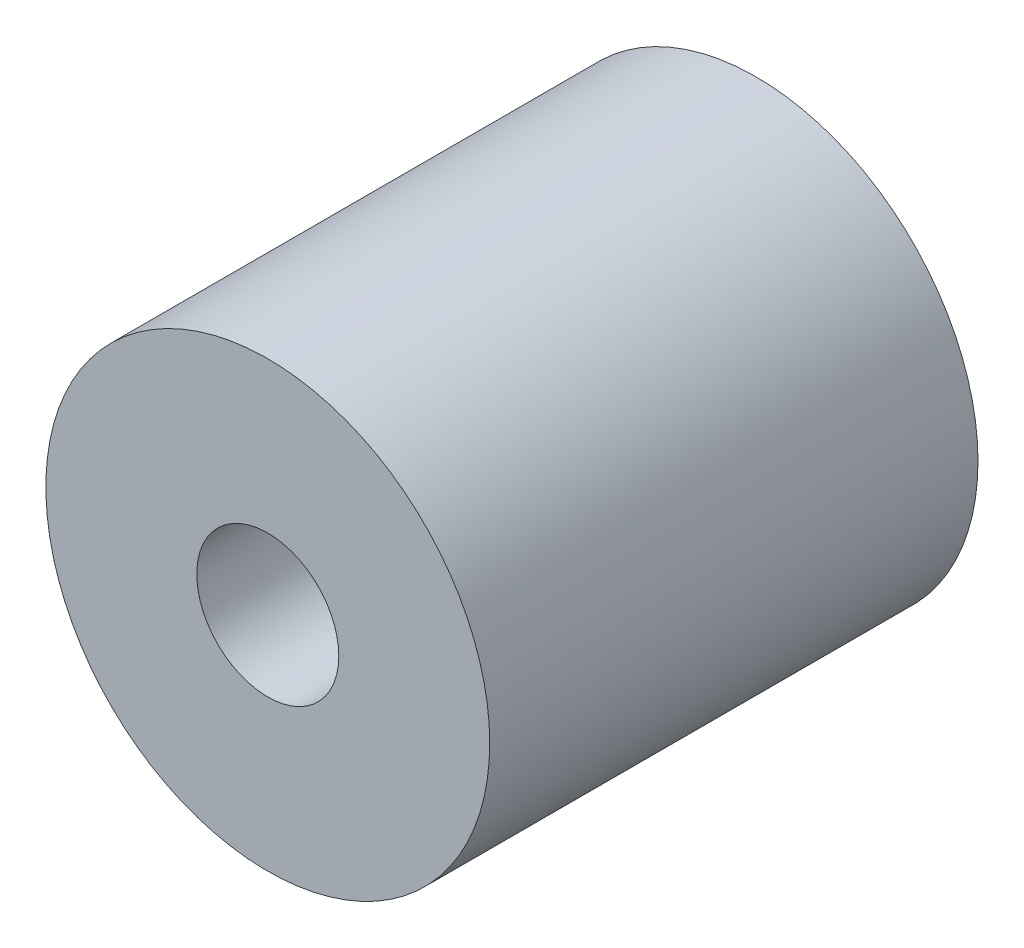
SolidWorks part; units mm, degrees
ref_plane "前视基准面" through (0, 0, 0) normal (0, 0, 1) x (1, 0, 0)
ref_plane "上视基准面" through (0, 0, 0) normal (0, 1, 0) x (1, 0, 0)
ref_plane "右视基准面" through (0, 0, 0) normal (1, 0, 0) x (0, 0, -1)
other "Configuration Table"
sketch "草图1" plane through (0, 0, 0) normal (0, 0, 1) x (1, 0, 0)
  circle A0 centre (0, 0) radius 10
  circle A1 centre (0, 0) radius 3.2
  point P0 (0, 0)
  dimension "D1" = 6.4
  dimension "D2" = 20
extrude "凸台-拉伸1" add sketch "草图1" against normal mid plane 22
